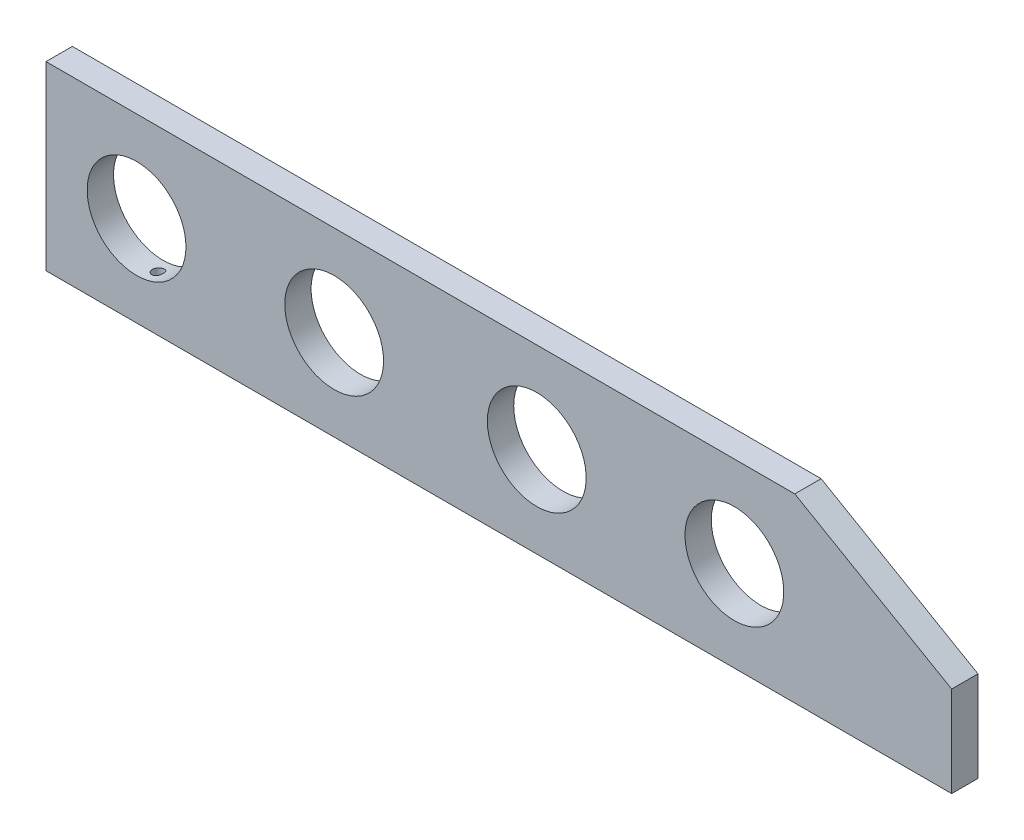
SolidWorks part; units mm, degrees
material "S45C"
ref_plane "前视" through (0, 0, 0) normal (0, 0, 1) x (1, 0, 0)
ref_plane "上视" through (0, 0, 0) normal (0, 1, 0) x (1, 0, 0)
ref_plane "右视" through (0, 0, 0) normal (1, 0, 0) x (0, 0, -1)
sketch "草图1" plane through (0, 0, 0) normal (0, 0, 1) x (1, 0, 0)
  line L1 (-275, -55) -> (275, -55)
  line L2 (-275, -55) -> (-275, 55)
  line L3 (-275, 55) -> (275, 55)
  line L4 (275, -55) -> (275, 55)
  line L5 (-275, -55) -> (275, 55) construction
  line L6 (-275, 55) -> (275, -55) construction
  point P0 (0, 0)
  dimension "D1" = 550
  dimension "D2" = 110
extrude "凸台-拉伸1" add sketch "草图1" along normal mid plane 16
sketch "草图2" plane through (0, 0, 8) normal (0, 0, 1) x (1, 0, 0)
  line L0 (-260, 39) -> (255, -40)
  line L1 (275, 55) -> (-275, 55) construction
  line L2 (275, -55) -> (275, 55) construction
  line L3 (275, -40) -> (275, 55)
  line L4 (275, 55) -> (-260, 55)
  line L5 (-275, 55) -> (-275, -55) construction
  line L6 (-275, -55) -> (275, -55) construction
  line L7 (-260, 55) -> (-260, 39)
  line L8 (275, -40) -> (255, -40)
  dimension "D1" = 15
  dimension "D2" = 15
  dimension "D3" = 16
  dimension "D4" = 20
extrude "切除-拉伸1" [suppressed] cut sketch "草图2" against normal through all
sketch "草图3" [suppressed] plane through (0, 0, 8) normal (0, 0, 1) x (1, 0, 0)
  line L0 (-165, -55) -> (165, -55) construction
  line L1 (-165, 55) -> (-165, -55) construction
  line L2 (-150, 39) -> (145, -40) construction
  line L3 (34.3315, -31.0681) -> (-142.4826, 16.2821)
  line L5 (-145, 14.3502) -> (-145, -33)
  line L6 (-143, -35) -> (33.8141, -35)
  arc A0 (-142.4826, 16.2821) -> (-145, 14.3502) centre (-143, 14.3502) ccw
  arc A1 (34.3315, -31.0681) -> (33.8141, -35) centre (33.8141, -33) cw
  arc A2 (-145, -33) -> (-143, -35) centre (-143, -33) ccw
  dimension "D1" = 20
  dimension "D2" = 20
  dimension "D3" = 2
  dimension "D4" = 2
  dimension "D5" = 20
extrude "切除-拉伸2" [suppressed] cut sketch "草图3" against normal through all
ref_plane "基准面1" through (-255, 0, 0) normal (-1, 0, 0) x (0, 0, 1)
ref_plane "基准面2" through (0, -25, 0) normal (0, -1, 0) x (1, 0, 0)
fillet "圆角1" [suppressed] radius 4
chamfer "倒角1" [suppressed] distance 0.3 angle 45
hole_wizard "打孔尺寸(%根据)内六角圆柱头螺钉的类型2" positions "草图4" profile "草图5" counterbore size "M5" standard "GB"
sketch "草图4" [suppressed] plane through (-150, 0, 0) normal (1, 0, 0) x (0, 0, -1)
  line L0 (0, -54.7) -> (0, 67.6049) construction
  line L1 (-7.7, -54.7) -> (7.7, -54.7) construction
  line L3 (-7.7, 55) -> (7.7, 55) construction
  line L4 (7.7, -55) -> (-7.7, -55) construction
  point P0 (0, 48)
  point P2 (0, -27)
  dimension "D1" = 7
  dimension "D2" = 28
sketch "草图5" plane through (-150, 48, 0) normal (0, 1, 0) x (0, 0, -1)
  line L0 (0, 0) -> (0, 15)
  line L1 (0, 15) -> (2.75, 15)
  line L3 (2.75, 15) -> (2.75, 5.7)
  line L4 (2.75, 5.7) -> (5, 5.7)
  line L5 (5, 5.7) -> (5, 0)
  line L7 (5, 0) -> (0, 0)
  line L11 (0, -6.35) -> (0, 107.95) construction
  dimension "通孔孔直径" = 5.5
  dimension "通孔孔深度" = 15
  dimension "柱形沉头孔直径" = 10
  dimension "柱形沉头孔深度" = 5.7
hole_wizard "打孔尺寸(%根据)内六角圆柱头螺钉的类型2" positions "草图6" profile "草图7" counterbore size "M5" standard "GB"
sketch "草图6" [suppressed] plane through (0, -35, 0) normal (0, 1, 0) x (1, 0, 0)
  line L1 (165, 7.7) -> (165, -7.7) construction
  line L2 (-147.1123, 8) -> (144.414, 8) construction
  point P4 (155, 0)
  point P18 (25, 0)
  point P20 (-105, 0)
  dimension "D1" = 8
  dimension "D2" = 130
  dimension "D3" = 10
  dimension "D4" = 130
sketch "草图7" plane through (155, -35, 0) normal (1, 0, 0) x (0, 0, 1)
  line L0 (0, 0) -> (0, 20)
  line L1 (0, 20) -> (2.75, 20)
  line L3 (2.75, 20) -> (2.75, 5.7)
  line L4 (2.75, 5.7) -> (5, 5.7)
  line L5 (5, 5.7) -> (5, 0)
  line L7 (5, 0) -> (0, 0)
  line L11 (0, -6.35) -> (0, 107.95) construction
  dimension "通孔孔直径" = 5.5
  dimension "通孔孔深度" = 20
  dimension "柱形沉头孔直径" = 10
  dimension "柱形沉头孔深度" = 5.7
sketch "草图8" [suppressed] plane through (0, -35, 0) normal (0, 1, 0) x (1, 0, 0)
  circle A0 centre (25, 0) radius 5 construction
  circle A1 centre (-105, 0) radius 5 construction
  circle A2 centre (25, 0) radius 5
  circle A3 centre (-105, 0) radius 5
extrude "切除-拉伸3" [suppressed] cut sketch "草图8" along normal through all
sketch "草图9" plane through (0, 0, 8) normal (0, 0, 1) x (1, 0, 0)
  line L0 (179.7372, 55) -> (275, 0)
  line L1 (275, 55) -> (-275, 55) construction
  line L5 (275, -55) -> (275, 55) construction
  dimension "D1" = 30
extrude "切除-拉伸4" cut sketch "草图9" against normal through all and the other way through all
hole_wizard "Hole1" positions "Point_Sketch" profile "Profil_Sketch" tap size "M8" standard "ISO"
sketch "Point_Sketch" plane through (-134.2135, -55, 9.1678) normal (0, -1, 0) x (1, 0, 0)
  point P0 (-80.7865, -9.1678)
  point P2 (119.2135, -9.1678)
  point P4 (369.2135, -9.1678)
sketch "Profil_Sketch" plane through (-215, -55, 0) normal (1, 0, 0) x (0, 0, -1)
  line L0 (0, 0) -> (0, 28.0279)
  line L1 (0, 28.0279) -> (3.375, 26)
  line L2 (3.375, 26) -> (3.375, 0)
  line L5 (3.375, 0) -> (0, 0)
  line L10 (0, 28.0279) -> (-3.375, 26) construction
  line L11 (0, -6.35) -> (0, 107.95) construction
  dimension "Tap Drill Dia." = 6.75
  dimension "Tap Drill Depth" = 26
  dimension "Drill Angle" = 118
cosmetic thread "孔螺蚊线1" parameters "D1"=18, "D2"=8
cosmetic thread "孔螺蚊线2" parameters "D1"=18, "D2"=8
cosmetic thread "孔螺蚊线3" parameters "D1"=18, "D2"=8
cosmetic thread "装饰螺纹线1" parameters "D1"=18, "D2"=8
cosmetic thread "装饰螺纹线2" parameters "D1"=18, "D2"=8
cosmetic thread "装饰螺纹线3" parameters "D1"=18, "D2"=8
other "usin_TS240_M8x25-SH<1>"
hole_wizard "Hole11" positions "Point_Sketch1" profile "Profil_Sketch1" tap size "M8" standard "ISO"
sketch "Point_Sketch1" plane through (-275, -17.8322, -14.2135) normal (-1, 0, 0) x (0, 0, 1)
  point P0 (14.2135, -9.1678)
  point P2 (14.2135, 62.8322)
sketch "Profil_Sketch1" plane through (-275, -27, 0) normal (0, 1, 0) x (0, 0, 1)
  line L0 (0, 0) -> (0, 30.0279)
  line L1 (0, 30.0279) -> (3.375, 28)
  line L2 (3.375, 28) -> (3.375, 0)
  line L5 (3.375, 0) -> (0, 0)
  line L10 (0, 30.0279) -> (-3.375, 28) construction
  line L11 (0, -6.35) -> (0, 107.95) construction
  dimension "Tap Drill Dia." = 6.75
  dimension "Tap Drill Depth" = 28
  dimension "Drill Angle" = 118
cosmetic thread "孔螺蚊线4" parameters "D1"=20, "D2"=8
cosmetic thread "孔螺蚊线5" parameters "D1"=20, "D2"=8
other "usin_TS240_M8x22-SH<2>"
sketch "草图10" plane through (0, 0, 8) normal (0, 0, 1) x (1, 0, 0)
  line L0 (-38.4808, 30) -> (-38.4808, 96.7774) construction
  line L1 (173.0385, 30) -> (173.0385, -30) construction
  line L5 (173.0385, 30) -> (-250, 30)
  line L6 (173.0385, 30) -> (-250, 30) construction
  line L7 (250, -30) -> (250, -14.4338)
  line L8 (250, -30) -> (250, -14.4338) construction
  line L10 (250, -14.4338) -> (173.0385, 30)
  line L11 (-250, 30) -> (-250, -30)
  line L12 (-250, -30) -> (250, -30)
  line L13 (250, -14.4338) -> (173.0385, 30) construction
  line L14 (-250, 30) -> (-250, -30) construction
  line L15 (-250, -30) -> (250, -30) construction
  circle A0 centre (-220, 0) radius 30
  circle A1 centre (-100, 0) radius 30
  circle A2 centre (23.0385, 0) radius 30
  circle A3 centre (143.0385, 0) radius 30
  dimension "D2" = 120
  dimension "D1" = 25
extrude "切除-拉伸5" cut sketch "草图10" against normal through all
